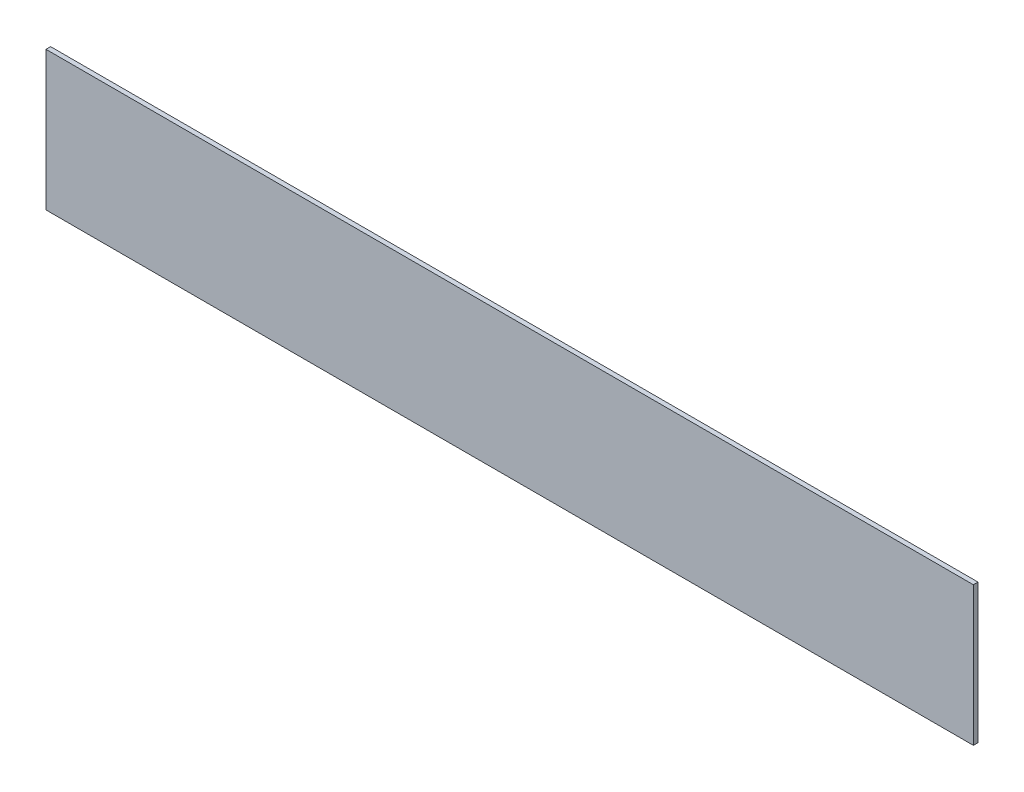
SolidWorks part; units mm, degrees
ref_plane "Front Plane" through (0, 0, 0) normal (0, 0, 1) x (1, 0, 0)
ref_plane "Top Plane" through (0, 0, 0) normal (0, 1, 0) x (1, 0, 0)
ref_plane "Right Plane" through (0, 0, 0) normal (1, 0, 0) x (0, 0, -1)
sketch "Sketch1" plane through (0, 0, 0) normal (0, 0, 1) x (1, 0, 0)
  line L0 (1000, 0) -> (-1000, 0) construction
  line L1 (1000, 150) -> (-1000, 150)
  line L2 (1000, 150) -> (1000, -150)
  line L3 (1000, -150) -> (-1000, -150)
  line L4 (-1000, 150) -> (-1000, -150)
  line L5 (1000, 150) -> (-1000, -150) construction
  line L6 (1000, -150) -> (-1000, 150) construction
  point P0 (0, 0)
  dimension "D1" = 2000
  dimension "D2" = 300
extrude "Boss-Extrude1" add sketch "Sketch1" along normal blind 10
